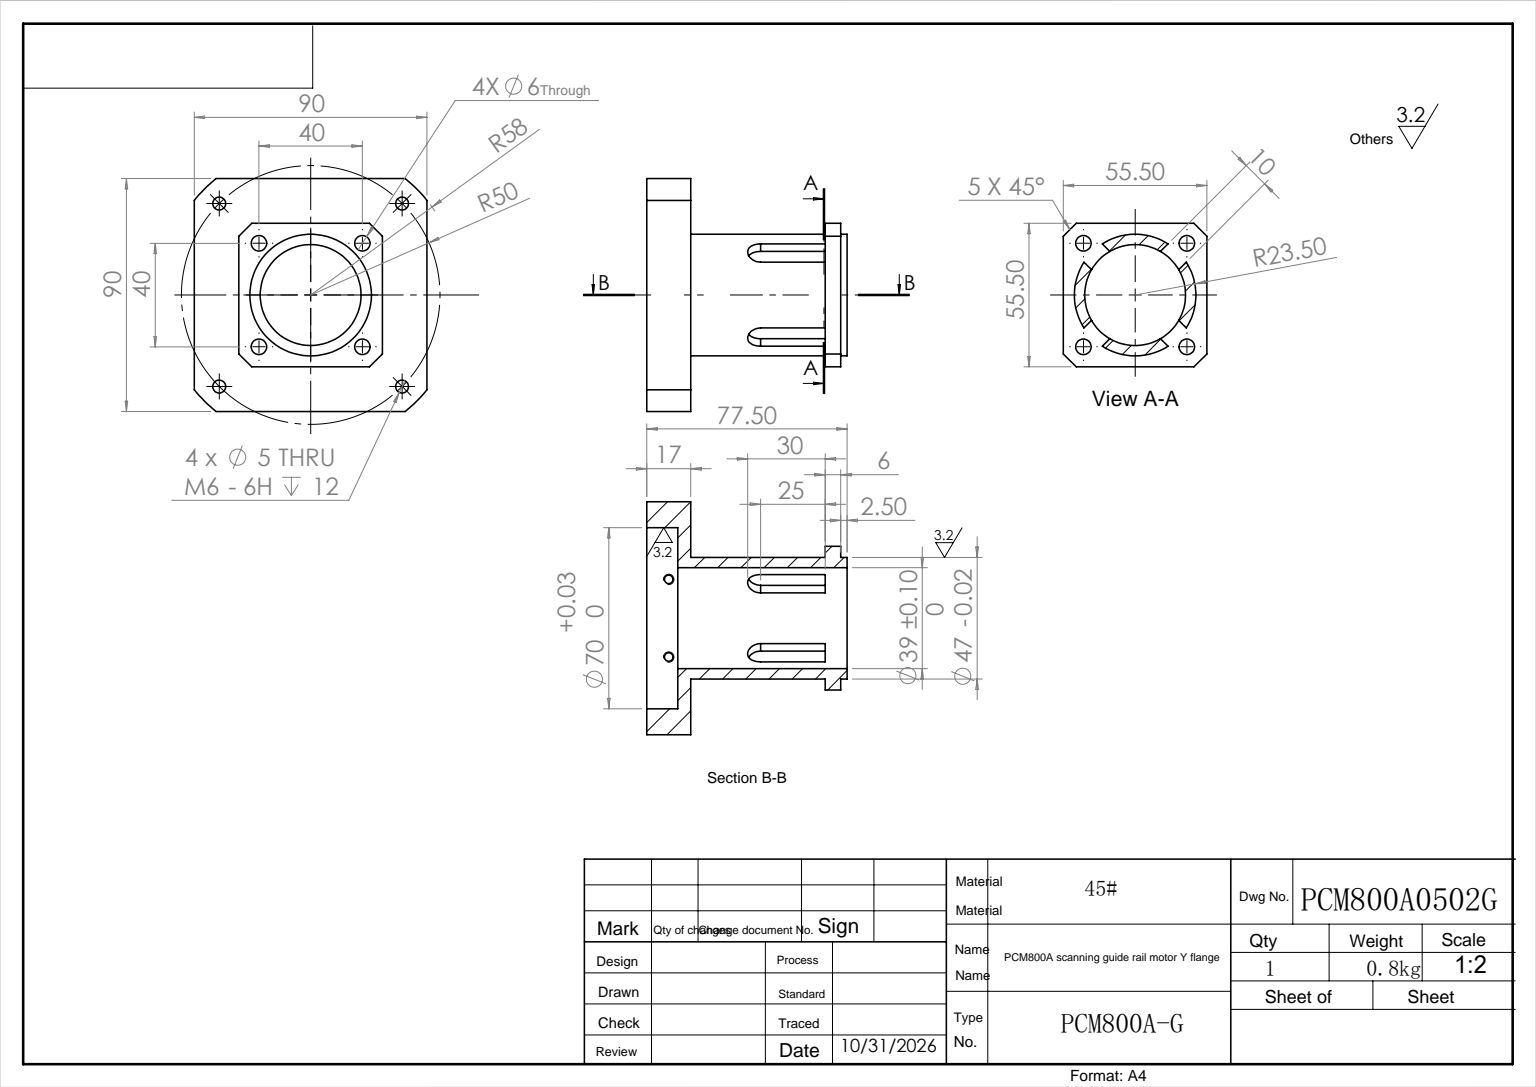
SolidWorks part; units mm, degrees
ref_plane "前视" through (0, 0, 0) normal (0, 0, 1) x (1, 0, 0)
ref_plane "上视" through (0, 0, 0) normal (0, 1, 0) x (1, 0, 0)
ref_plane "右视" through (0, 0, 0) normal (1, 0, 0) x (0, 0, -1)
sketch "草图1" plane through (0, 0, 0) normal (0, 0, 1) x (1, 0, 0)
  line L1 (0, 0) -> (90, 0)
  line L2 (0, 0) -> (0, 90)
  line L3 (0, 90) -> (90, 90)
  line L4 (90, 0) -> (90, 90)
  dimension "D1" = 90
  dimension "D2" = 90
extrude "拉伸1" add sketch "草图1" along normal blind 17
sketch "草图2" plane through (0, 0, 0) normal (0, 0, -1) x (-1, 0, 0)
  line L0 (-90, 45) -> (0, 45) construction
  line L1 (-90, 0) -> (-90, 90) construction
  line L2 (0, 90) -> (0, 0) construction
  line L3 (-45, 90) -> (-45, 0) construction
  line L4 (-90, 90) -> (0, 90) construction
  line L5 (0, 0) -> (-90, 0) construction
  circle A0 centre (-45, 45) radius 23.5
  dimension "D1" = 47
extrude "拉伸2" add sketch "草图2" along normal blind 52
sketch "草图3" plane through (0, 0, -52) normal (0, 0, -1) x (-1, 0, 0)
  line L0 (-45, 90) -> (-45, 0) construction
  line L1 (-90, 90) -> (0, 90) construction
  line L2 (0, 0) -> (-90, 0) construction
  line L3 (-90, 45) -> (0, 45) construction
  line L4 (-72.75, 72.75) -> (-17.25, 72.75)
  line L5 (-72.75, 72.75) -> (-72.75, 17.25)
  line L6 (-72.75, 17.25) -> (-17.25, 17.25)
  line L7 (-17.25, 72.75) -> (-17.25, 17.25)
  line L8 (-90, 0) -> (-90, 90) construction
  line L9 (0, 90) -> (0, 0) construction
  dimension "D1" = 55.5
  dimension "D2" = 27.75
  dimension "D3" = 27.75
  dimension "D4" = 55.5
extrude "拉伸3" add sketch "草图3" along normal blind 6
sketch "草图4" plane through (0, 0, -58) normal (0, 0, -1) x (-1, 0, 0)
  line L0 (-72.75, 45) -> (-17.25, 45) construction
  line L1 (-72.75, 72.75) -> (-72.75, 17.25) construction
  line L2 (-17.25, 17.25) -> (-17.25, 72.75) construction
  line L3 (-45, 72.75) -> (-45, 17.25) construction
  line L4 (-17.25, 72.75) -> (-72.75, 72.75) construction
  line L5 (-72.75, 17.25) -> (-17.25, 17.25) construction
  circle A0 centre (-45, 45) radius 23.5
  dimension "D1" = 47
extrude "拉伸4" add sketch "草图4" along normal blind 2.5
sketch "草图5" plane through (0, 0, -60.5) normal (0, 0, -1) x (-1, 0, 0)
  circle A0 centre (-45, 45) radius 19.5
  circle A1 centre (-45, 45) radius 23.5 construction
  dimension "D1" = 39
extrude "切除-拉伸1" cut sketch "草图5" against normal through all
sketch "草图6" plane through (0, 0, 17) normal (0, 0, 1) x (1, 0, 0)
  line L0 (0, 45) -> (90, 45) construction
  line L1 (0, 90) -> (0, 0) construction
  line L2 (90, 0) -> (90, 90) construction
  line L3 (45, 90) -> (45, 0) construction
  line L4 (90, 90) -> (0, 90) construction
  line L5 (0, 0) -> (90, 0) construction
  line L6 (0, 90) -> (90, 0) construction
  line L7 (0, 0) -> (90, 90) construction
hole_wizard "M6 螺纹孔1" positions "3D草图1" profile "草图7" tap size "M6" standard "GB" end condition up to next
sketch3d "3D草图1"
  line L0 (0, 90, 17) -> (90, 0, 17) construction
  line L1 (0, 0, 17) -> (90, 90, 17) construction
  point P0 (9.6447, 80.3553, 17)
  point P5 (80.3553, 80.3553, 17)
  point P6 (9.6447, 9.6447, 17)
  point P7 (80.3553, 9.6447, 17)
  dimension "D1" = 50
  dimension "D2" = 50
  dimension "D3" = 50
  dimension "D4" = 50
sketch "草图7" plane through (9.6447, 80.3553, 17) normal (1, 0, 0) x (0, -1, 0)
  line L0 (0, 0) -> (0, 17)
  line L1 (0, 17) -> (2.5, 17)
  line L3 (2.5, 17) -> (2.5, 12)
  line L4 (2.5, 12) -> (3, 12)
  line L5 (3, 12) -> (3, 0)
  line L7 (3, 0) -> (0, 0)
  line L11 (0, -6.35) -> (0, 107.95) construction
  dimension "籵謂蹟恇謂郰芛眻噤" = 5
  dimension "籵謂蹟恇謂郰芛旮僅" = 17
  dimension "蹟恇盄翋眻噤" = 6
  dimension "蹟恇盄旮僅" = 12
sketch "草图8" plane through (0, 0, 17) normal (0, 0, 1) x (1, 0, 0)
  line L0 (0, 45) -> (90, 45) construction
  circle A0 centre (45, 45) radius 35
  dimension "D1" = 70
extrude "切除-拉伸2" cut sketch "草图8" against normal blind 12
sketch "草图9" plane through (0, 0, 17) normal (0, 0, 1) x (1, 0, 0)
  line L0 (0, 45) -> (90, 45) construction
  circle A0 centre (45, 45) radius 58
  dimension "D1" = 116
extrude "切除-拉伸3" cut sketch "草图9" against normal through all flip side to cut
sketch "草图10" plane through (0, 0, -58) normal (0, 0, -1) x (-1, 0, 0)
  line L0 (-72.75, 45) -> (-17.25, 45) construction
  line L1 (-72.75, 72.75) -> (-72.75, 17.25) construction
  line L2 (-17.25, 17.25) -> (-17.25, 72.75) construction
  line L3 (-45, 72.75) -> (-45, 17.25) construction
  line L4 (-17.25, 72.75) -> (-72.75, 72.75) construction
  line L5 (-72.75, 17.25) -> (-17.25, 17.25) construction
  line L6 (-45, 45) -> (-72.75, 72.75) construction
  circle A0 centre (-65, 65) radius 3
  circle A1 centre (-25, 65) radius 3
  circle A2 centre (-25, 25) radius 3
  circle A3 centre (-65, 25) radius 3
  dimension "D1" = 6
  dimension "D2" = 20
extrude "切除-拉伸4" cut sketch "草图10" against normal blind 12
chamfer "倒角1" distance 5 angle 45 4 edges at (17.25, 17.25, -55) (17.25, 72.75, -55) (72.75, 17.25, -55) (72.75, 72.75, -55)
ref_plane "基准面1" through (-25.9571, 25.9571, 0) normal (-0.7071, 0.7071, 0) x (0, 0, 1)
sketch "草图11" plane through (-25.9571, 25.9571, 0) normal (-0.7071, 0.7071, 0) x (0, 0, 1)
  line L0 (-52, 63.6396) -> (22.725, 63.6396) construction
  line L1 (-52, 67.1751) -> (-52, 60.1041) construction
  line L2 (-52, 27.9307) -> (-52, 60.1041) construction
  line L3 (-52, 58.6396) -> (-27, 58.6396)
  line L4 (-52, 58.6396) -> (-52, 68.6396)
  line L5 (-52, 68.6396) -> (-27, 68.6396)
  arc A0 (-27, 68.6396) -> (-27, 58.6396) centre (-27, 63.6396) cw
  dimension "D1" = 25
  dimension "D2" = 5
extrude "切除-拉伸5" cut sketch "草图11" against normal through all
ref_plane "基准面2" through (70.9571, 70.9571, 0) normal (0.7071, 0.7071, 0) x (-0.7071, 0.7071, 0)
sketch "草图12" plane through (70.9571, 70.9571, 0) normal (0.7071, 0.7071, 0) x (-0.7071, 0.7071, 0)
  line L0 (0, -52) -> (0, 36.5134) construction
  line L1 (-3.5355, -52) -> (3.5355, -52) construction
  line L2 (-3.5355, -52) -> (-35.7089, -52) construction
  line L3 (-5, -52) -> (5, -52)
  line L4 (-5, -52) -> (-5, -27)
  line L6 (5, -52) -> (5, -27)
  arc A0 (-5, -27) -> (5, -27) centre (0, -27) cw
  dimension "D1" = 10
  dimension "D2" = 5
  dimension "D3" = 25
extrude "切除-拉伸6" cut sketch "草图12" against normal through all
ref_plane "基准面3" through (45, 0, 0) normal (1, 0, 0) x (0, 0, -1)
hole_wizard "M4 螺纹孔1" positions "草图15" profile "草图14" tap size "M4" standard "GB"
sketch "草图15" plane through (0, 0, 0) normal (0, -1, 0) x (1, 0, 0)
  line L0 (-4.4525, 8.5) -> (96.7778, 8.5) construction
  line L2 (8.4077, 17) -> (81.5923, 17) construction
  line L3 (45, 17) -> (45, -22.5469) construction
  point P0 (60, 8.5)
  point P1 (30, 8.5)
  dimension "D1" = 8.5
  dimension "D2" = 15
  dimension "D3" = 15
sketch "草图14" plane through (60, 0, 8.5) normal (1, 0, 0) x (0, 0, -1)
  line L0 (0, 0) -> (0, 13.3772)
  line L1 (0, 13.3772) -> (1.65, 13.3772)
  line L2 (1.65, 13.3772) -> (1.65, 0)
  line L5 (1.65, 0) -> (0, 0)
  line L11 (0, -6.35) -> (0, 107.95) construction
  dimension "通孔螺纹孔钻头直径" = 3.3
  dimension "通孔螺纹孔钻头深度" = 13.3772
cosmetic thread "孔螺蚊线3" parameters "D2"=4
cosmetic thread "孔螺蚊线4" parameters "D2"=4
